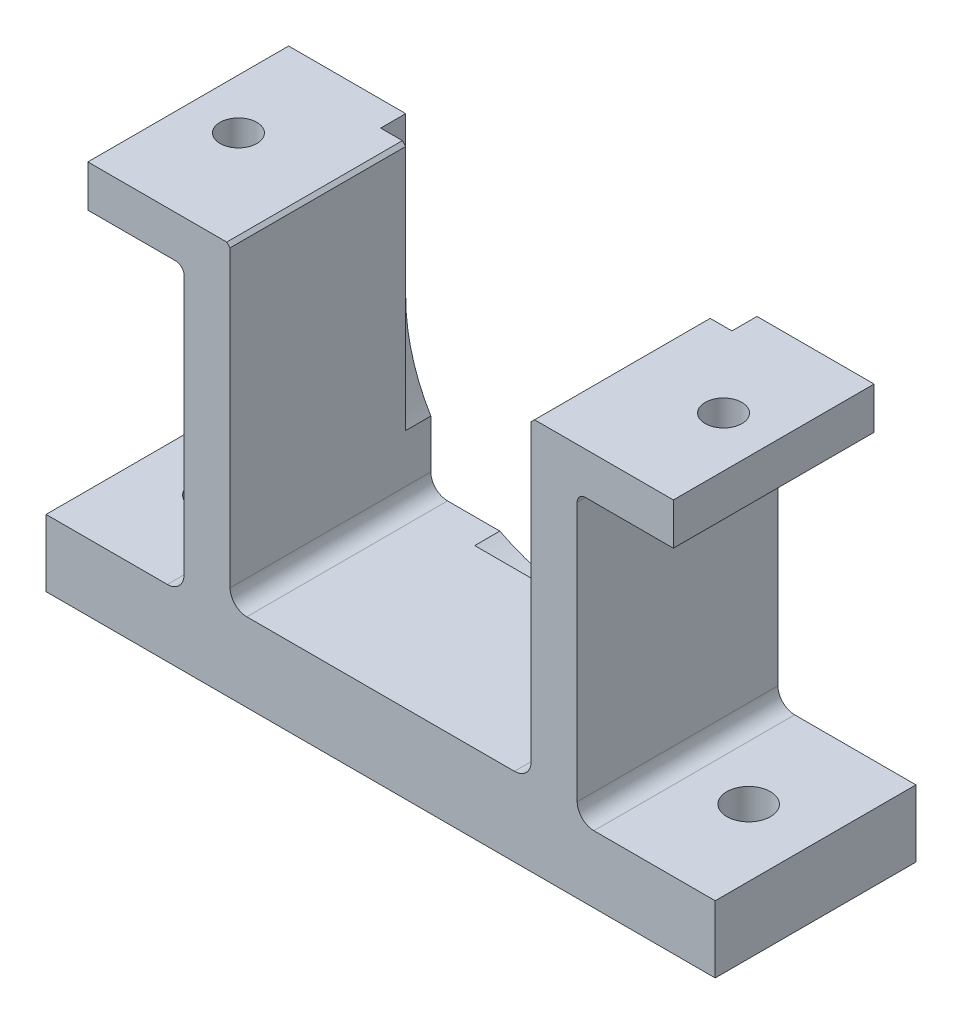
from build123d import *

# Parameters (mm, degrees)
BOSS_EXTRUDE1_DEPTH = 60
SKETCH2_R           = 13
CUT_EXTRUDE1_DEPTH  = 87
SKETCH3_R           = 11
CUT_EXTRUDE2_DEPTH  = 87
CUT_EXTRUDE3_DEPTH  = 15


with BuildPart() as part:
    # Sketch1 → Boss-Extrude1 (new, symmetric)
    with BuildSketch(Plane.XY):
        with BuildLine():
            Line((-200, 0), (200, 0))
            Line((200, 0), (200, 40))
            Line((200, 40), (127.5, 40))
            ThreePointArc((127.5, 40), (120.428932188, 42.928932188), (117.5, 50))
            Line((117.5, 50), (117.5, 205))
            ThreePointArc((117.5, 205), (118.964466094, 208.535533906), (122.5, 210))
            Line((122.5, 210), (175, 210))
            Line((175, 210), (175, 235))
            Line((175, 235), (92, 235))
            Line((92, 235), (90, 233))
            Line((90, 233), (90, 57))
            ThreePointArc((90, 57), (87.071067812, 49.928932188), (80, 47))
            Line((80, 47), (-80, 47))
            ThreePointArc((-80, 47), (-87.071067812, 49.928932188), (-90, 57))
            Line((-90, 57), (-90, 233))
            Line((-90, 233), (-92, 235))
            Line((-92, 235), (-175, 235))
            Line((-175, 235), (-175, 210))
            Line((-175, 210), (-122.5, 210))
            ThreePointArc((-122.5, 210), (-118.964466094, 208.535533906), (-117.5, 205))
            Line((-117.5, 205), (-117.5, 50))
            ThreePointArc((-117.5, 50), (-120.428932188, 42.928932188), (-127.5, 40))
            Line((-127.5, 40), (-200, 40))
            Line((-200, 40), (-200, 0))
        make_face()
    extrude(amount=BOSS_EXTRUDE1_DEPTH, both=True)

    # Sketch2 → Cut-Extrude1 (cut)
    with BuildSketch(Plane.XZ):
        with Locations(Location((-160, 0, 0), (0, 0, 270))):
            Circle(SKETCH2_R)
        with Locations(Location((160, 0, 0), (0, 0, 270))):
            Circle(SKETCH2_R)
    extrude(amount=-CUT_EXTRUDE1_DEPTH, mode=Mode.SUBTRACT)

    # Sketch3 → Cut-Extrude2 (cut)
    with BuildSketch(Plane(origin=(0, 235, 0), x_dir=(1, 0, 0), z_dir=(0, 1, 0))):
        with Locations(Location((-145, 0, 0), (0, 0, 270))):
            Circle(SKETCH3_R)
        with Locations(Location((145, 0, 0), (0, 0, 180))):
            Circle(SKETCH3_R)
    extrude(amount=-CUT_EXTRUDE2_DEPTH, mode=Mode.SUBTRACT)

    # Sketch4 → Cut-Extrude3 (cut)
    with BuildSketch(Plane(origin=(0, 0, -60), x_dir=(-1, 0, 0), z_dir=(0, 0, -1))):
        with BuildLine():
            Line((-105, 140), (-105, 340))
            Line((-105, 340), (105, 340))
            Line((105, 340), (105, 140))
            ThreePointArc((105, 140), (0, 35), (-105, 140))
        make_face()
    extrude(amount=-CUT_EXTRUDE3_DEPTH, mode=Mode.SUBTRACT)


solid = part.part
